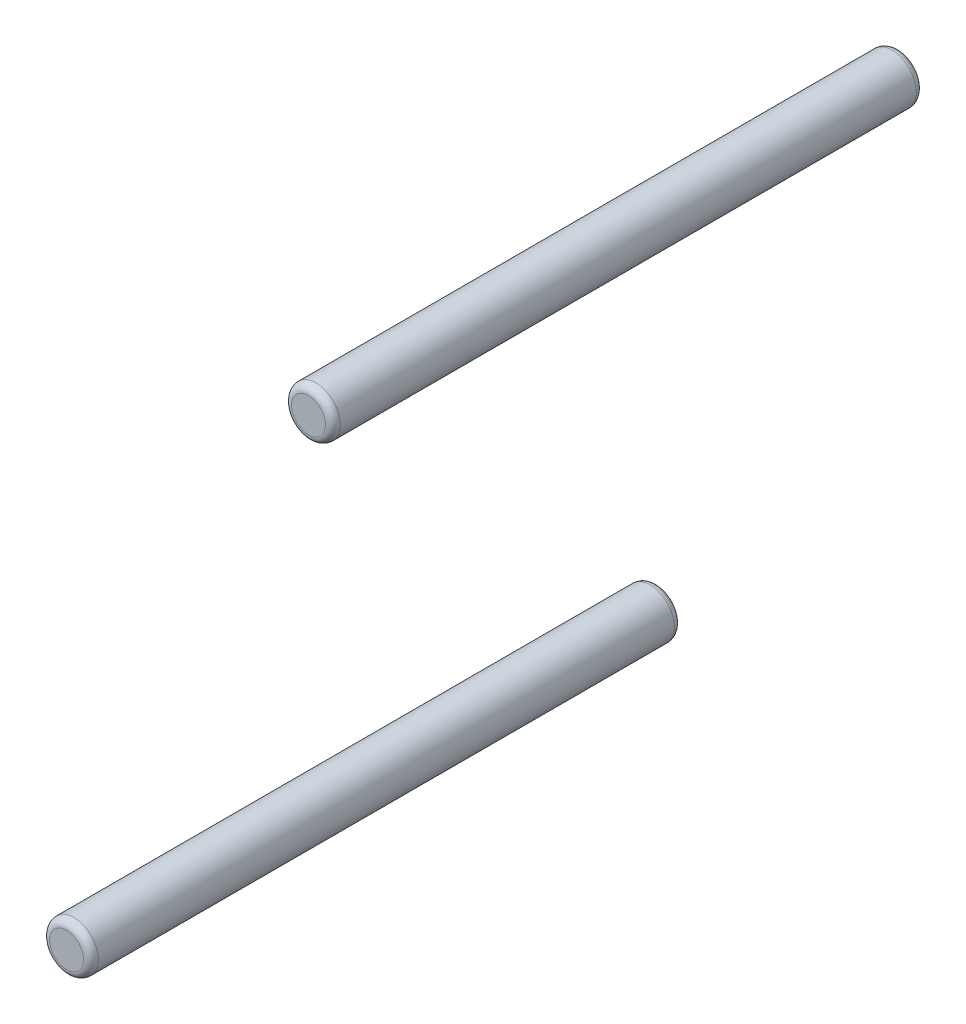
SolidWorks part; units mm, degrees
ref_plane "Front Plane" through (0, 0, 0) normal (0, 0, 1) x (1, 0, 0)
ref_plane "Top Plane" through (0, 0, 0) normal (0, 1, 0) x (1, 0, 0)
ref_plane "Right Plane" through (0, 0, 0) normal (1, 0, 0) x (0, 0, -1)
sketch "Sketch1" plane through (0, 0, 0) normal (0, 0, 1) x (1, 0, 0)
  circle A0 centre (-16.3789, -39.542) radius 3.3
  circle A1 centre (16.3789, 39.542) radius 3.3
  dimension "D1" = 6.6
  dimension "D2" = 6.6
extrude "Boss-Extrude1" add sketch "Sketch1" along normal blind 80
fillet "Fillet1" radius 1 2 edges at (-13.0789, -39.542, 80) (-13.0789, -39.542, 0)
fillet "Fillet2" radius 1 2 edges at (19.6789, 39.542, 80) (19.6789, 39.542, 0)
